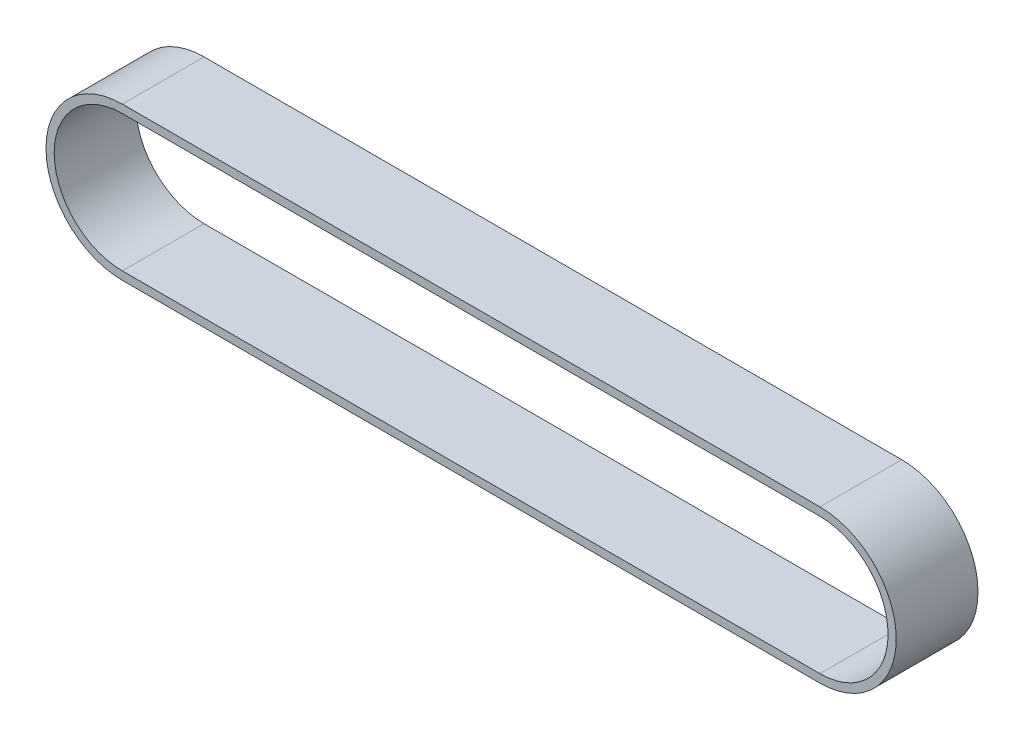
SolidWorks part; units mm, degrees
ref_plane "前视基准面" through (0, 0, 0) normal (0, 0, 1) x (1, 0, 0)
ref_plane "上视基准面" through (0, 0, 0) normal (0, 1, 0) x (1, 0, 0)
ref_plane "右视基准面" through (0, 0, 0) normal (1, 0, 0) x (0, 0, -1)
sketch "草图1" plane through (0, 0, 0) normal (0, 0, 1) x (1, 0, 0)
  line L0 (-128, 0) -> (128, 0) construction
  line L1 (-128, 25) -> (128, 25)
  line L2 (-128, -25) -> (128, -25)
  arc A0 (-128, 25) -> (-128, -25) centre (-128, 0) ccw
  arc A1 (128, -25) -> (128, 25) centre (128, 0) ccw
  point P2 (0, 0)
  dimension "D2" = 25
  dimension "D1" = 256
extrude "拉伸-薄壁1" add sketch "草图1" along normal blind 30 thin thin type one direction wall 3
